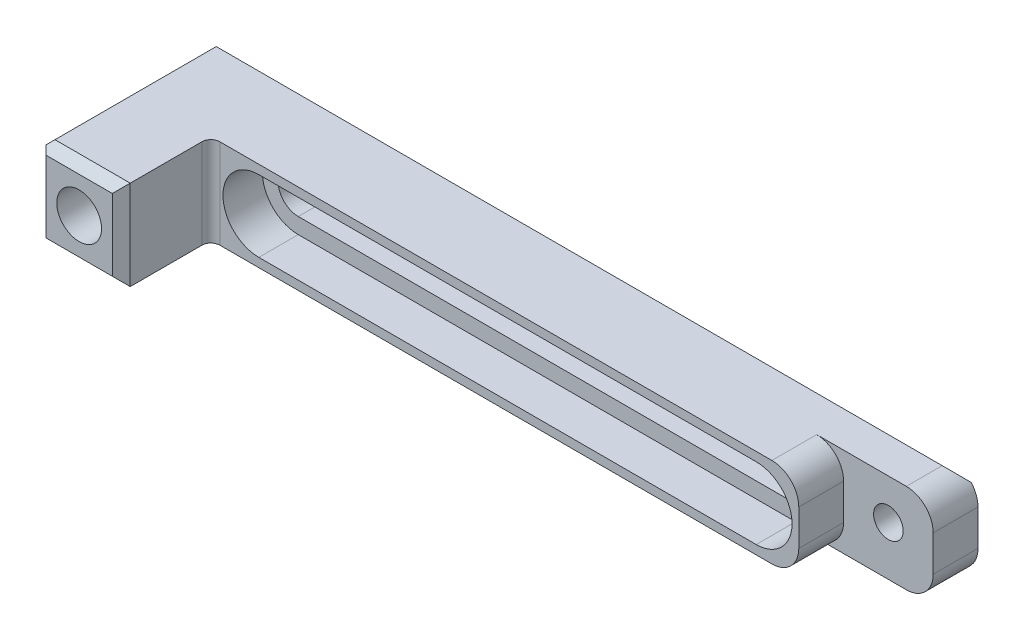
SolidWorks part; units mm, degrees
ref_plane "Front Plane" through (0, 0, 0) normal (0, 0, 1) x (1, 0, 0)
ref_plane "Top Plane" through (0, 0, 0) normal (0, 1, 0) x (1, 0, 0)
ref_plane "Right Plane" through (0, 0, 0) normal (1, 0, 0) x (0, 0, -1)
sketch "Sketch1" plane through (0, 0, 0) normal (0, 1, 0) x (1, 0, 0)
  line L1 (42.5, -5) -> (-42.5, -5)
  line L2 (42.5, -5) -> (42.5, 5)
  line L3 (42.5, 5) -> (-42.5, 5)
  line L4 (-42.5, -5) -> (-42.5, 5)
  line L5 (42.5, -5) -> (-42.5, 5) construction
  line L6 (42.5, 5) -> (-42.5, -5) construction
  point P0 (0, 0)
  dimension "D1" = 85
  dimension "D2" = 10
extrude "Boss-Extrude1" add sketch "Sketch1" along normal blind 10
sketch "Sketch2" plane through (0, 0, 5) normal (0, 0, 1) x (1, 0, 0)
  line L0 (0, 10) -> (0, 0) construction
  line L1 (-42.5, 10) -> (42.5, 10) construction
  line L2 (-27.75, 5) -> (27.75, 5) construction
  line L3 (-27.75, 9) -> (27.75, 9)
  line L4 (-27.75, 1) -> (27.75, 1)
  arc A0 (-27.75, 9) -> (-27.75, 1) centre (-27.75, 5) ccw
  arc A1 (27.75, 1) -> (27.75, 9) centre (27.75, 5) ccw
  point P7 (0, 5)
  dimension "D2" = 4
  dimension "D1" = 55.5
extrude "Cut-Extrude1" cut sketch "Sketch2" against normal blind 4.4
sketch "Sketch3" plane through (0, 0, 0.6) normal (0, 0, 1) x (1, 0, 0)
  line L0 (-27.75, 5) -> (27.75, 5) construction
  line L1 (-27.75, 7.25) -> (27.75, 7.25)
  line L2 (-27.75, 2.75) -> (27.75, 2.75)
  arc A0 (-27.75, 7.25) -> (-27.75, 2.75) centre (-27.75, 5) ccw
  arc A1 (27.75, 2.75) -> (27.75, 7.25) centre (27.75, 5) ccw
  point P4 (0, 5)
  dimension "D1" = 2.25
extrude "Cut-Extrude2" cut sketch "Sketch3" against normal through all
sketch "Sketch4" plane through (0, 0, 5) normal (0, 0, 1) x (1, 0, 0)
  line L0 (-42.5, 0) -> (42.5, 0) construction
  line L1 (-42.5, 10) -> (-33.1, 10)
  line L2 (-42.5, 10) -> (-42.5, 0)
  line L3 (-42.5, 0) -> (-33.1, 0)
  line L4 (-33.1, 10) -> (-33.1, 0)
  dimension "D1" = 9.4
extrude "Boss-Extrude2" add sketch "Sketch4" along normal blind 10 contours L4 L3 L2 L1
sketch "Sketch5" plane through (0, 0, 5) normal (0, 0, 1) x (1, 0, 0)
  line L0 (-33.1, 0) -> (42.5, 0) construction
  line L1 (42.5, 10) -> (32.5, 10)
  line L2 (42.5, 10) -> (42.5, 0)
  line L3 (42.5, 0) -> (32.5, 0)
  line L4 (32.5, 10) -> (32.5, 0)
  dimension "D1" = 10
extrude "Cut-Extrude3" cut sketch "Sketch5" against normal blind 5
hole_wizard "M6 Tapped Hole1" positions "Sketch6" profile "Sketch7" tap size "M6" standard "GB"
sketch "Sketch6" plane through (0, 0, 15) normal (0, 0, 1) x (1, 0, 0)
  point P0 (-37.8, 5)
sketch "Sketch7" plane through (-37.8, 5, 15) normal (1, 0, 0) x (0, -1, 0)
  line L0 (0, 0) -> (0, 18.5022)
  line L1 (0, 18.5022) -> (2.5, 17)
  line L2 (2.5, 17) -> (2.5, 0)
  line L5 (2.5, 0) -> (0, 0)
  line L10 (0, 18.5022) -> (-2.5, 17) construction
  line L11 (0, -6.35) -> (0, 107.95) construction
  dimension "螺纹孔钻头直径" = 5
  dimension "螺纹孔钻头深度" = 17
  dimension "导头角度" = 118
cosmetic thread "HoleThreadLine1"
hole_wizard "M4 Tapped Hole1" positions "Sketch8" profile "Sketch9" tap size "M4" standard "GB"
sketch "Sketch8" plane through (0, 0, 0) normal (0, 0, 1) x (1, 0, 0)
  line L0 (42.5, 0) -> (42.5, 10) construction
  line L1 (42.5, 10) -> (32.5, 10) construction
  point P0 (37.5, 5.5)
  point P3 (37.5, 5.5)
  dimension "D1" = 5
  dimension "D2" = 4.5
sketch "Sketch9" plane through (37.5, 5.5, 0) normal (1, 0, 0) x (0, -1, 0)
  line L0 (0, 0) -> (0, 12.4914)
  line L1 (0, 12.4914) -> (1.65, 11.5)
  line L2 (1.65, 11.5) -> (1.65, 0)
  line L5 (1.65, 0) -> (0, 0)
  line L10 (0, 12.4914) -> (-1.65, 11.5) construction
  line L11 (0, -6.35) -> (0, 107.95) construction
  dimension "螺纹孔钻头直径" = 3.3
  dimension "螺纹孔钻头深度" = 11.5
  dimension "导头角度" = 118
cosmetic thread "HoleThreadLine2"
fillet "Fillet1" radius 3 2 edges at (32.5, 0, 2.5) (32.5, 10, 2.5)
chamfer "Chamfer1" [suppressed] distance 2 angle 45
chamfer "Chamfer2" distance 1 angle 45 4 edges at (-42.5, 5, 15) (-37.8, 10, 15) (-33.1, 5, 15) (-37.8, 0, 15)
fillet "Fillet2" radius 1 1 edges at (-33.1, 5, 5)
chamfer "Chamfer3" distance 1 angle 45 5 edges at (0, 10, -5) (0, 0, -5) (-42.5, 10, 4.5) (-42.5, 5, -5) (-42.5, 0, 4.5)
fillet "Fillet3" radius 3 2 edges at (42.5, 0, -2) (42.5, 10, -2)
equation "\"1\"= \"代号代号\""
equation "\"2\"= \"名称代号\""
